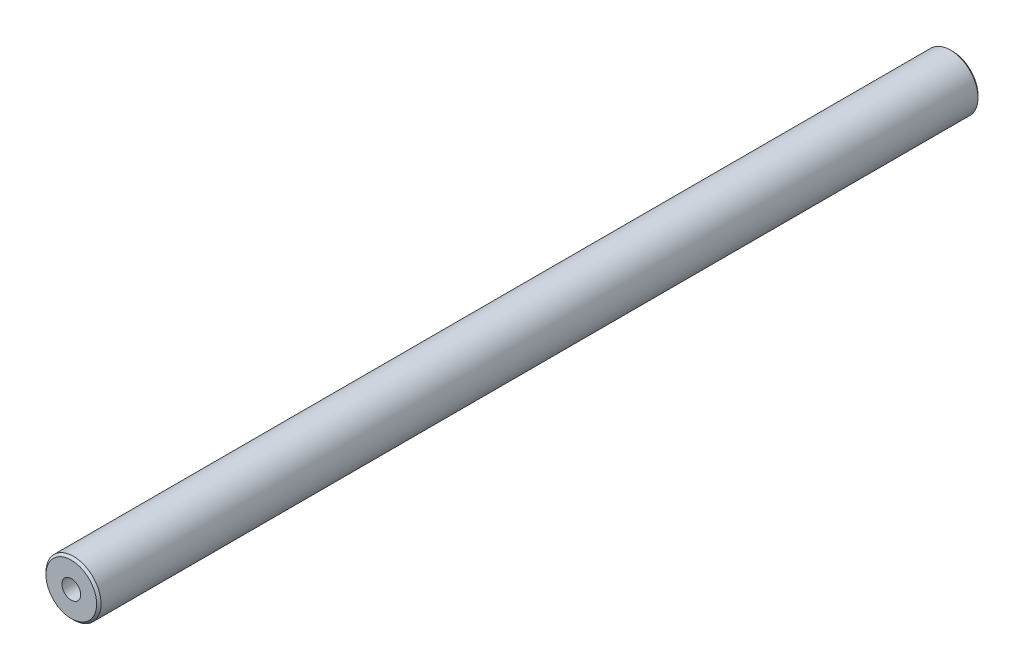
SolidWorks part; units mm, degrees
material "45"
ref_plane "前视基准面" through (0, 0, 0) normal (0, 0, 1) x (1, 0, 0)
ref_plane "上视基准面" through (0, 0, 0) normal (0, 1, 0) x (1, 0, 0)
ref_plane "右视基准面" through (0, 0, 0) normal (1, 0, 0) x (0, 0, -1)
sketch "草图1" plane through (0, 0, 0) normal (0, 0, 1) x (1, 0, 0)
  circle A0 centre (0, 0) radius 12.5
  dimension "D1" = 25
extrude "凸台-拉伸1" add sketch "草图1" along normal mid plane 400
chamfer "倒角1" distance 1 angle 45 2 edges at (12.5, 0, -200) (12.5, 0, 200)
hole_wizard "M10 螺纹孔1" positions "草图2" profile "草图3" tap size "M10" standard "GB"
sketch "草图2" plane through (0, 0, 200) normal (0, 0, 1) x (1, 0, 0)
  point P0 (0, 0)
sketch "草图3" plane through (0, 0, 200) normal (1, 0, 0) x (0, -1, 0)
  line L0 (0, 0) -> (0, 27.0537)
  line L1 (0, 27.0537) -> (4.25, 24.5)
  line L2 (4.25, 24.5) -> (4.25, 0)
  line L5 (4.25, 0) -> (0, 0)
  line L10 (0, 27.0537) -> (-4.25, 24.5) construction
  line L11 (0, -6.35) -> (0, 107.95) construction
  dimension "螺纹孔钻头直径" = 8.5
  dimension "螺纹孔钻头深度" = 24.5
  dimension "导头角度" = 118
cosmetic thread "孔螺蚊线1"
